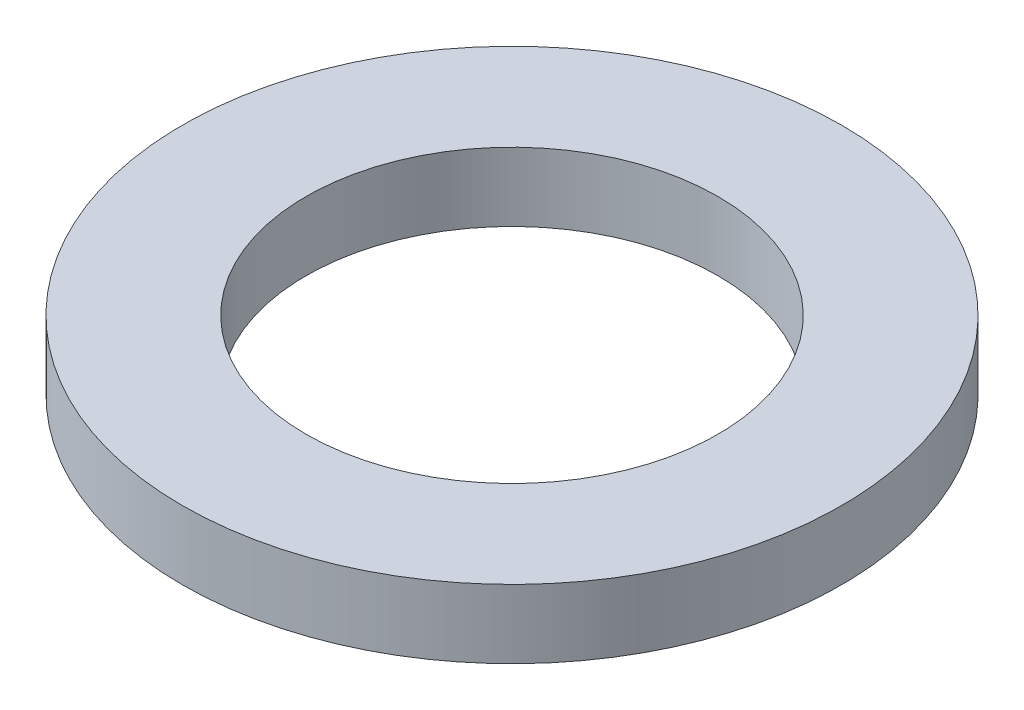
SolidWorks part; units mm, degrees
material "Q235"
ref_plane "Plane1" through (0, 0, 0) normal (0, 0, 1) x (1, 0, 0)
ref_plane "Plane2" through (0, 0, 0) normal (0, 1, 0) x (1, 0, 0)
ref_plane "Plane3" through (0, 0, 0) normal (1, 0, 0) x (0, 0, -1)
sketch "Dimension Sketch" plane through (0, 0, 0) normal (0, 0, 1) x (1, 0, 0)
  line L0 (0, 0) -> (24, 0) construction
  point P3 (2.5, 0)
  point P4 (24, 0)
  point P5 (15, 0)
  dimension "h" = 2.5
  dimension "d2" = 24
  dimension "d1" = 15
sketch "Sketch1" plane through (0, 0, 0) normal (0, 0, 1) x (1, 0, 0)
  line L0 (0, 0) -> (0, 52.7318) construction
  line L2 (-7.5, 8.6445) -> (-12, 8.6445)
  line L3 (-7.5, 8.6445) -> (-7.5, 11.1445)
  line L4 (-7.5, 11.1445) -> (-12, 11.1445)
  line L5 (-12, 8.6445) -> (-12, 11.1445)
  dimension "D1" = 7.5
  dimension "D2" = 12
  dimension "h" = 2.5
revolve "Boss-Revolve" add sketch "Sketch1" angle 360 about L0
